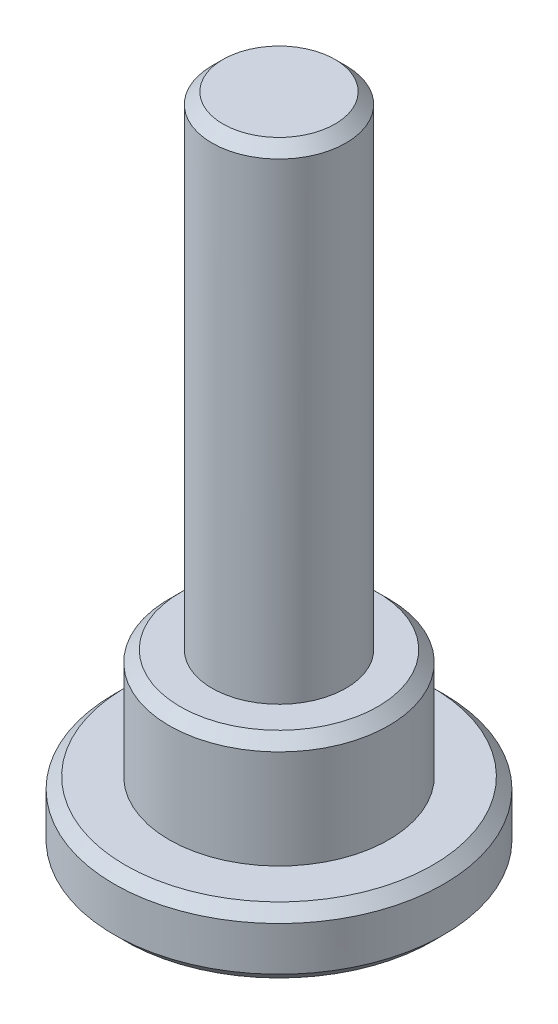
from build123d import *

# Parameters (mm, degrees)
CHAMFER1_SIZE = 0.5


with BuildPart() as part:
    # Sketch1 → Revolve1 (revolve)
    with BuildSketch(Plane(origin=(0, 0, 0), x_dir=(0, 0, -1), z_dir=(1, 0, 0))):
        Polygon((0, 30), (3.05, 30), (3.05, 8), (5, 8), (5, 3), (7.5, 3), (7.5, 0), (0, 0), align=None)
    revolve(axis=Axis((0, 0, 0), (0, 1, 0)))

    # Chamfer1
    chamfer1_edges = [part.edges().sort_by_distance(p)[0] for p in [
        (0, 0, 7.5),
        (0, 3, 7.5),
        (0, 8, 5),
        (0, 30, 3.05),
    ]]
    chamfer(chamfer1_edges, length=CHAMFER1_SIZE)


solid = part.part
